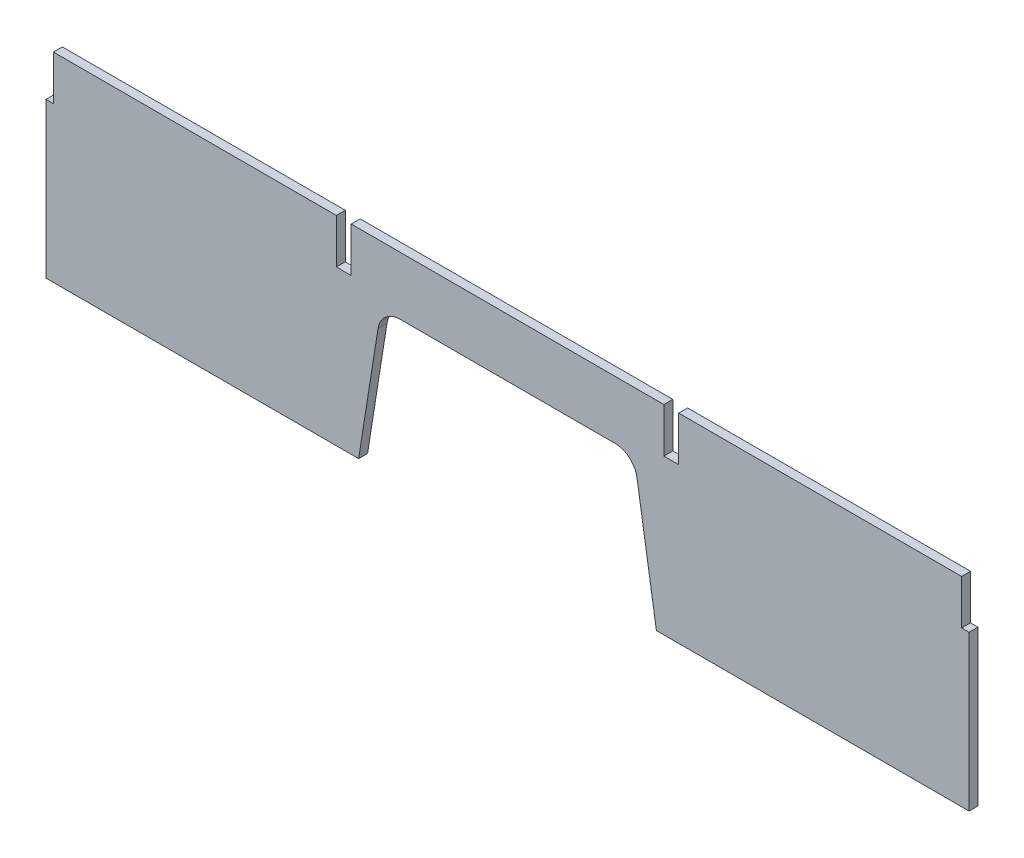
from build123d import *

# Parameters (mm, degrees)
BOSS_EXTRUDE1_DEPTH = 12


with BuildPart() as part:
    # Sketch1 → Boss-Extrude1 (new body)
    with BuildSketch(Plane.XY):
        with BuildLine():
            Line((0, 0), (420, 0))
            Line((420, 0), (446.084814008, 164.693033951))
            ThreePointArc((446.084814008, 164.693033951), (456.232022776, 182.812178968), (475.715464226, 190))
            Line((475.715464226, 190), (764.284535774, 190))
            ThreePointArc((764.284535774, 190), (783.767977224, 182.812178968), (793.915185992, 164.693033951))
            Line((793.915185992, 164.693033951), (820, 0))
            Line((820, 0), (1240, 0))
            Line((1240, 0), (1240, 208))
            Line((1240, 208), (1230, 208))
            Line((1230, 208), (1230, 268))
            Line((1230, 268), (850, 268))
            Line((850, 268), (850, 208))
            Line((850, 208), (830, 208))
            Line((830, 208), (830, 268))
            Line((830, 268), (410, 268))
            Line((410, 268), (410, 208))
            Line((410, 208), (390, 208))
            Line((390, 208), (390, 268))
            Line((390, 268), (10, 268))
            Line((10, 268), (10, 208))
            Line((10, 208), (0, 208))
            Line((0, 208), (0, 0))
        make_face()
    extrude(amount=BOSS_EXTRUDE1_DEPTH)


solid = part.part
